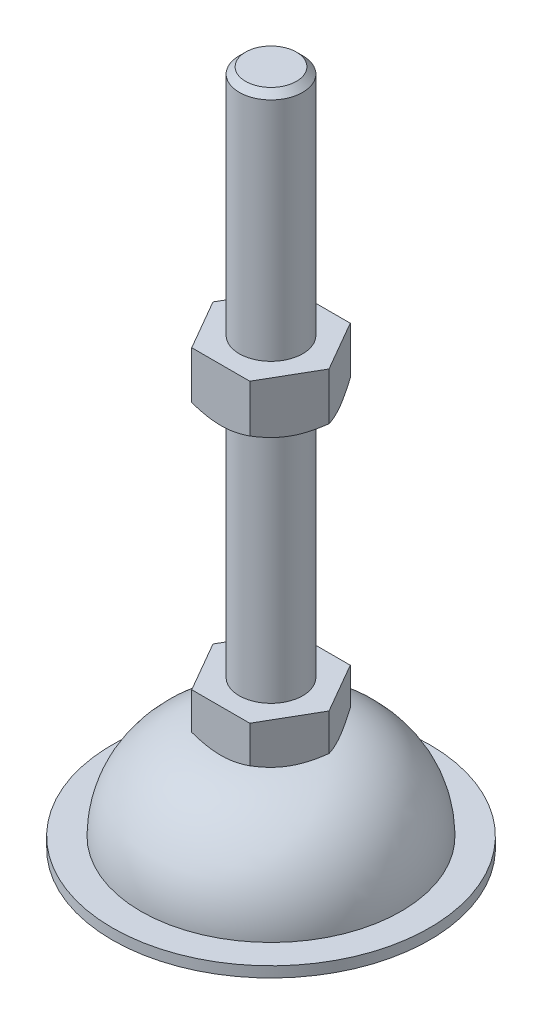
from build123d import *

# Parameters (mm, degrees)
CHAMFER1_SIZE       = 1.2
BOSS_EXTRUDE1_START = 20
BOSS_EXTRUDE1_DEPTH = 8
BOSS_EXTRUDE2_START = 74
BOSS_EXTRUDE2_DEPTH = 10
SKETCH5_R           = 12.439310229
SKETCH5_R_2         = 9.5
CUT_EXTRUDE1_DEPTH  = 6.4
CUT_EXTRUDE1_TAPER  = 55
SKETCH6_R           = 12.439310229
SKETCH6_R_2         = 9.5
CUT_EXTRUDE4_DEPTH  = 5
CUT_EXTRUDE4_DRAFT  = -55


with BuildPart() as part:
    # Sketch2 → Revolve1 (revolve)
    with BuildSketch(Plane(origin=(0, 0, 0), x_dir=(0, 0, -1), z_dir=(1, 0, 0)), mode=Mode.PRIVATE) as revolve1_sk:
        with BuildLine():
            Line((0, 128), (6, 128))
            Line((6, 128), (6, 20))
            Line((6, 20), (6.6, 20))
            ThreePointArc((6.6, 20), (19.327922061, 14.727922061), (24.6, 2))
            Line((24.6, 2), (30, 2))
            Line((30, 2), (30, 0))
            Line((30, 0), (0, 0))
            Line((0, 0), (0, 128))
        make_face()
    revolve(revolve1_sk.sketch.rotate(Axis((0, 128, 0), (0, -1, 0)), 180), axis=Axis((0, 128, 0), (0, -1, 0)))

    # Chamfer1
    chamfer1_edges = [part.edges().sort_by_distance(p)[0] for p in [
        (0, 128, -6),
    ]]
    chamfer(chamfer1_edges, length=CHAMFER1_SIZE)

    # Sketch3 → Boss-Extrude1 (add)
    with BuildSketch(Plane(origin=(0, 0, 0), x_dir=(1, 0, 0), z_dir=(0, 1, 0)).offset(BOSS_EXTRUDE1_START)):
        Polygon((-10.969655115, 0), (-5.484827557, -9.5), (5.484827557, -9.5), (10.969655115, 0), (5.484827557, 9.5), (-5.484827557, 9.5), align=None)
    extrude(amount=BOSS_EXTRUDE1_DEPTH)

    # Sketch5 → Cut-Extrude1 (cut)
    with BuildSketch(Plane.XZ.offset(-20)):
        Circle(SKETCH5_R)
        Circle(SKETCH5_R_2, mode=Mode.SUBTRACT)
    extrude(amount=-CUT_EXTRUDE1_DEPTH, taper=CUT_EXTRUDE1_TAPER, mode=Mode.SUBTRACT)


with BuildPart() as body_2:
    # Sketch4 → Boss-Extrude2 (new body)
    with BuildSketch(Plane(origin=(0, 0, 0), x_dir=(1, 0, 0), z_dir=(0, 1, 0)).offset(BOSS_EXTRUDE2_START)):
        Polygon((-5.484827557, 9.5), (-10.969655115, 0), (-5.484827557, -9.5), (5.484827557, -9.5), (10.969655115, 0), (5.484827557, 9.5), align=None)
    extrude(amount=BOSS_EXTRUDE2_DEPTH)


with BuildPart() as cut_extrude4_tool:
    # Sketch6 → Cut-Extrude4 (with draft: the straight prism first)
    with BuildSketch(Plane.XZ.offset(-74)):
        Circle(SKETCH6_R)
        Circle(SKETCH6_R_2, mode=Mode.SUBTRACT)
    extrude(amount=-CUT_EXTRUDE4_DEPTH)
    # Cut-Extrude4: the draft: its side faces are tilted about the plane it starts from
    cut_extrude4_sides = [cut_extrude4_tool.faces().sort_by_distance(p)[0] for p in [
        (-12.439310229, 76.5, 0),
        (-9.5, 76.5, 0),
    ]]
    draft(cut_extrude4_sides, Plane.XZ.offset(-74), CUT_EXTRUDE4_DRAFT)


with BuildPart() as body_2_1:
    add(body_2.part)

    # Cut-Extrude4: cut by cut_extrude4_tool
    add(cut_extrude4_tool.part, mode=Mode.SUBTRACT)


solid = Compound([part.part, body_2_1.part])
